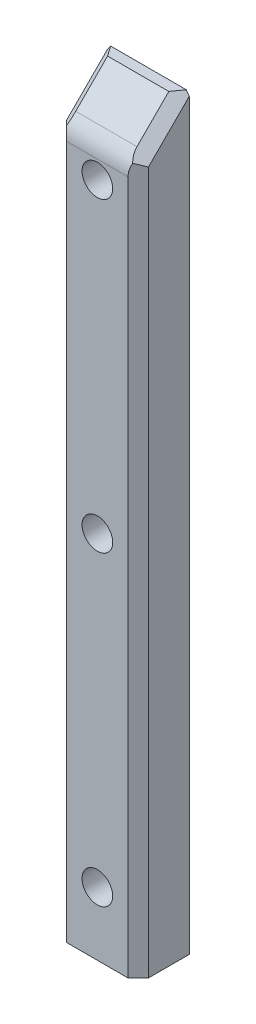
from build123d import *

# Parameters (mm, degrees)
SKETCH1_W                                          = 40
SKETCH1_H                                          = 366
BOSS_EXTRUDE1_DEPTH                                = 25
CHAMFER2_SIZE                                      = 20
SKETCH4_R                                          = 7.5
CUT_EXTRUDE1_DEPTH                                 = 2
HOLE_SIZE_BASED_ON_HEX_SOCKET_CAP_SCRE_D           = 9
HOLE_SIZE_BASED_ON_HEX_SOCKET_CAP_SCRE_CBORE_D     = 15
HOLE_SIZE_BASED_ON_HEX_SOCKET_CAP_SCRE_CBORE_DEPTH = 10
CHAMFER3_SIZE                                      = 5
CHAMFER4_SIZE                                      = 5
FILLET4_R                                          = 15


with BuildPart() as part:
    # Sketch1 → Boss-Extrude1 (new body)
    with BuildSketch(Plane.XY):
        Rectangle(SKETCH1_W, SKETCH1_H)
    extrude(amount=BOSS_EXTRUDE1_DEPTH)

    # Chamfer2
    chamfer2_edges = [part.edges().sort_by_distance(p)[0] for p in [
        (0, 183, 25),
    ]]
    chamfer(chamfer2_edges, length=CHAMFER2_SIZE)

    # Sketch4 → Cut-Extrude1 (cut)
    with BuildSketch(Plane.XY.offset(25)):
        with Locations((0, -152)):
            Circle(SKETCH4_R)
        with Locations((0, -2)):
            Circle(SKETCH4_R)
        with Locations((0, 148)):
            Circle(SKETCH4_R)
    extrude(amount=-CUT_EXTRUDE1_DEPTH, mode=Mode.SUBTRACT)

    # Hole Size (based on) hex socket cap screw type 1 (through all)
    with Locations(Plane.XY.offset(23)):
        with Locations((0, -152), (0, -2), (0, 148)):
            CounterBoreHole(HOLE_SIZE_BASED_ON_HEX_SOCKET_CAP_SCRE_D / 2, HOLE_SIZE_BASED_ON_HEX_SOCKET_CAP_SCRE_CBORE_D / 2, HOLE_SIZE_BASED_ON_HEX_SOCKET_CAP_SCRE_CBORE_DEPTH)

    # Chamfer3
    chamfer3_edges = [part.edges().sort_by_distance(p)[0] for p in [
        (-20, -10, 25),
        (20, -10, 25),
    ]]
    chamfer(chamfer3_edges, length=CHAMFER3_SIZE)

    # Chamfer4
    chamfer4_edges = [part.edges().sort_by_distance(p)[0] for p in [
        (20, 175.5, 12.5),
        (-20, 175.5, 12.5),
    ]]
    chamfer(chamfer4_edges, length=CHAMFER4_SIZE)

    # Fillet4
    fillet4_edges = [part.edges().sort_by_distance(p)[0] for p in [
        (0, 163, 25),
    ]]
    fillet(fillet4_edges, radius=FILLET4_R)


solid = part.part
